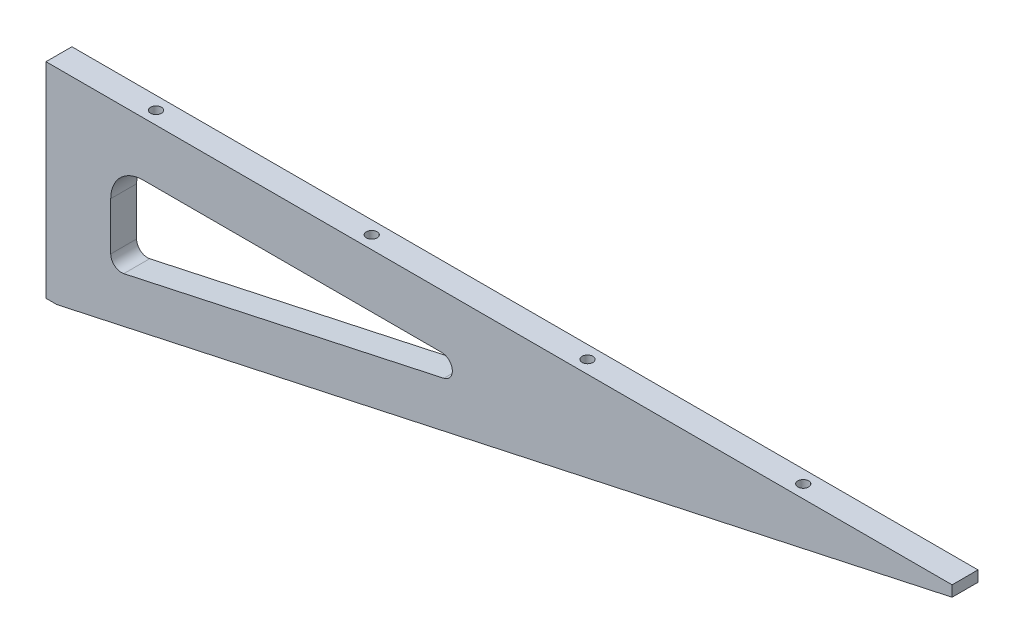
from build123d import *

# Parameters (mm, degrees)
BOSS_EXTRUDE1_DEPTH   = 12
M6_TAPPED_HOLE1_D     = 5
M6_TAPPED_HOLE1_DEPTH = 15
M6_TAPPED_HOLE1_TIP   = 1.502151548
M6_TAPPED_HOLE2_D     = 5
M6_TAPPED_HOLE2_DEPTH = 15
M6_TAPPED_HOLE2_TIP   = 1.502151548


with BuildPart() as part:
    # Sketch1 → Boss-Extrude1 (new body)
    with BuildSketch(Plane.XY):
        Polygon((0, -95), (0, 0), (420, 0), (420, -5), (5, -95), align=None)
        with BuildLine():
            Line((30, -62.172928769), (30, -40))
            ThreePointArc((30, -40), (34.393398282, -29.393398282), (45, -25))
            Line((45, -25), (183.352949325, -25))
            ThreePointArc((183.352949325, -25), (188.324471362, -29.467112929), (184.412653251, -34.886412548))
            Line((184.412653251, -34.886412548), (36.059703926, -67.059341317))
            ThreePointArc((36.059703926, -67.059341317), (31.861411116, -66.065133776), (30, -62.172928769))
        make_face(mode=Mode.SUBTRACT)
    extrude(amount=BOSS_EXTRUDE1_DEPTH)

    # M6 Tapped Hole1
    with Locations(Plane.ZY):
        with Locations((6, -15), (6, -47.5), (6, -80)):
            Hole(M6_TAPPED_HOLE1_D / 2, depth=M6_TAPPED_HOLE1_DEPTH)
            with Locations((0, 0, -(M6_TAPPED_HOLE1_DEPTH + M6_TAPPED_HOLE1_TIP / 2))):  # 118° drill point
                Cone(0, M6_TAPPED_HOLE1_D / 2, M6_TAPPED_HOLE1_TIP, mode=Mode.SUBTRACT)

    # M6 Tapped Hole2
    with Locations(Plane(origin=(0, 0, 0), x_dir=(-1, 0, 0), z_dir=(0, 1, 0))):
        with Locations((-45, 6), (-145, 6), (-245, 6), (-345, 6)):
            Hole(M6_TAPPED_HOLE2_D / 2, depth=M6_TAPPED_HOLE2_DEPTH)
            with Locations((0, 0, -(M6_TAPPED_HOLE2_DEPTH + M6_TAPPED_HOLE2_TIP / 2))):  # 118° drill point
                Cone(0, M6_TAPPED_HOLE2_D / 2, M6_TAPPED_HOLE2_TIP, mode=Mode.SUBTRACT)


solid = part.part
